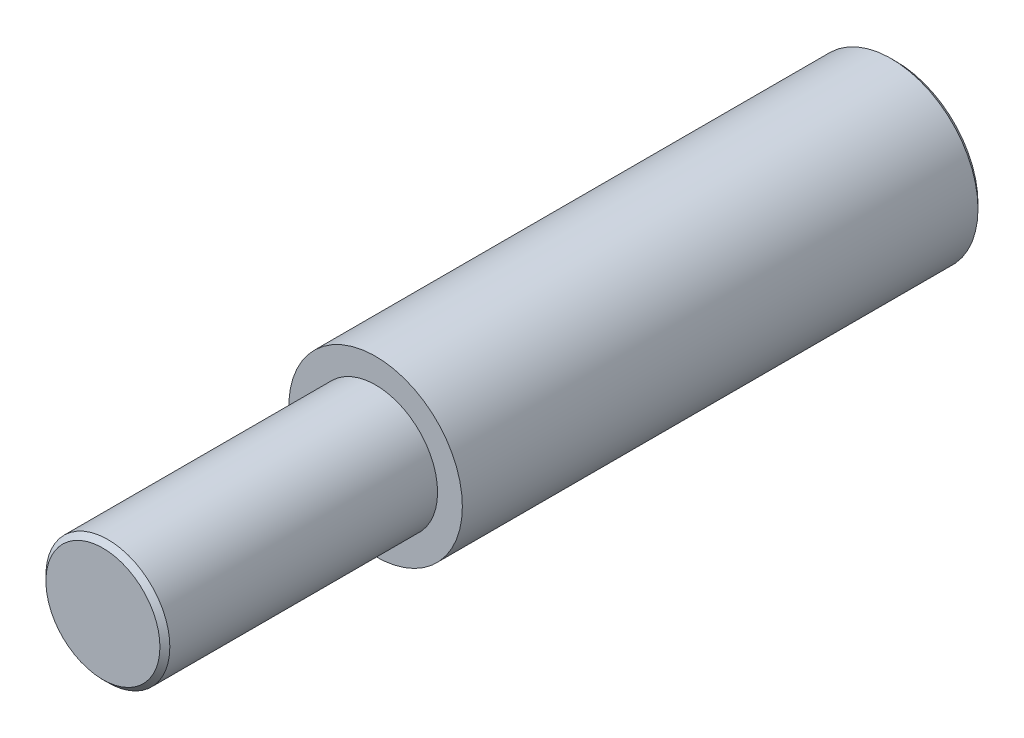
SolidWorks part; units mm, degrees
material "1023 碳钢板 (SS)"
ref_plane "Front Plane" through (0, 0, 0) normal (0, 0, 1) x (1, 0, 0)
ref_plane "Top Plane" through (0, 0, 0) normal (0, 1, 0) x (1, 0, 0)
ref_plane "Right Plane" through (0, 0, 0) normal (1, 0, 0) x (0, 0, -1)
sketch "Sketch1" plane through (0, 0, 0) normal (0, 0, 1) x (1, 0, 0)
  circle A0 centre (0, 0) radius 17.5
  dimension "D1" = 35
extrude "Boss-Extrude1" add sketch "Sketch1" along normal blind 105
sketch "Sketch2" plane through (0, 0, 105) normal (0, 0, 1) x (1, 0, 0)
  circle A0 centre (0, 0) radius 12.5
  dimension "D1" = 25
extrude "Boss-Extrude2" add sketch "Sketch2" along normal blind 55 contours A0
chamfer "Chamfer1" distance 1 angle 45 2 edges at (17.5, 0, 0) (12.5, 0, 160)
